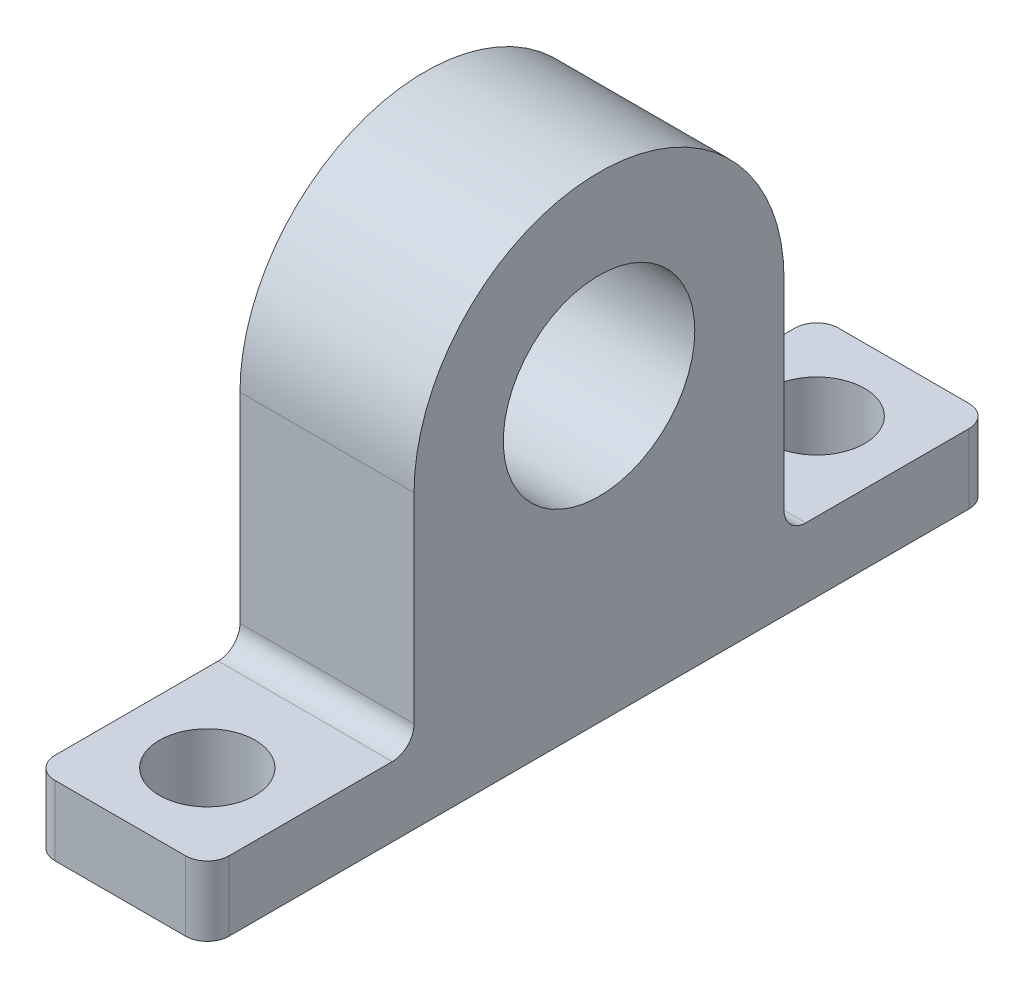
from build123d import *

# Parameters (mm, degrees)
SKETCH1_W           = 40
SKETCH1_H           = 180
SKETCH1_R           = 11
BOSS_EXTRUDE1_DEPTH = 16
SKETCH2_R           = 22
BOSS_EXTRUDE2_DEPTH = 20
FILLET1_R           = 5


with BuildPart() as part:
    # Sketch1 → Boss-Extrude1 (new body)
    with BuildSketch(Plane(origin=(0, 0, 0), x_dir=(1, 0, 0), z_dir=(0, 1, 0))):
        Rectangle(SKETCH1_W, SKETCH1_H)
        with Locations(Location((0, 70, 0), (0, 0, 270))):
            Circle(SKETCH1_R, mode=Mode.SUBTRACT)
        with Locations(Location((0, -70, 0), (0, 0, 90))):
            Circle(SKETCH1_R, mode=Mode.SUBTRACT)
    extrude(amount=BOSS_EXTRUDE1_DEPTH)

    # Sketch2 → Boss-Extrude2 (add, symmetric)
    with BuildSketch(Plane(origin=(0, 0, 0), x_dir=(0, 0, -1), z_dir=(1, 0, 0))):
        with BuildLine():
            Line((-42.5, 67), (-42.5, 16))
            Line((-42.5, 16), (42.5, 16))
            Line((42.5, 16), (42.5, 67))
            ThreePointArc((42.5, 67), (0, 109.5), (-42.5, 67))
        make_face()
        with Locations((0, 67)):
            Circle(SKETCH2_R, mode=Mode.SUBTRACT)
    extrude(amount=BOSS_EXTRUDE2_DEPTH, both=True)

    # Fillet1
    fillet1_edges = [part.edges().sort_by_distance(p)[0] for p in [
        (0, 16, 42.5),
        (20, 8, 90),
        (-20, 8, 90),
        (20, 8, -90),
        (-20, 8, -90),
        (0, 16, -42.5),
    ]]
    fillet(fillet1_edges, radius=FILLET1_R)


solid = part.part
